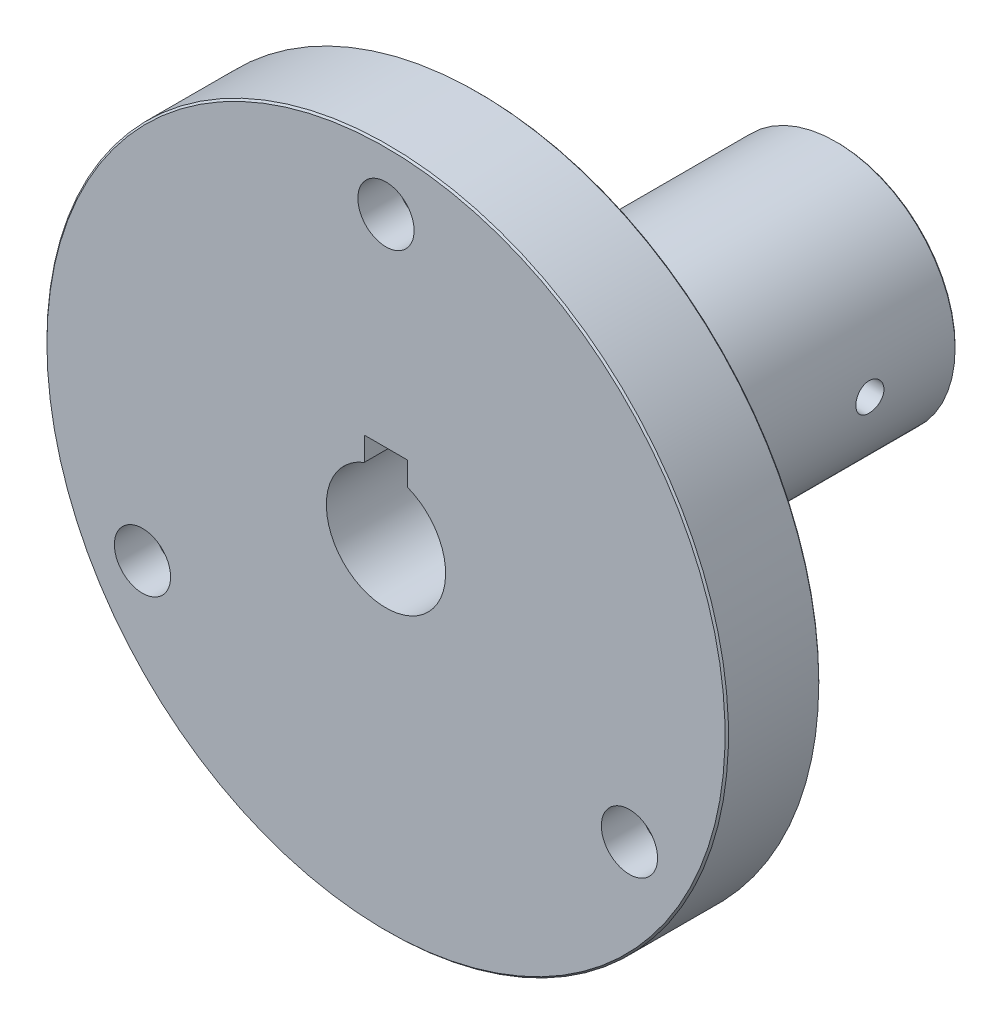
from build123d import *

# Parameters (mm, degrees)
SKETCH_1_R                   = 14
EXTRUDE_1_DEPTH              = 42
SKETCH_2_R                   = 40
EXTRUDE_2_DEPTH              = 11
SKETCH_3_R                   = 7
CUT_EXTRUDE_1_DEPTH          = 78.517739905
HOLE_WIZARD_M6_1_D           = 6.6
HOLE_WIZARD_M6_1_CBORE_D     = 11
HOLE_WIZARD_M6_1_CBORE_DEPTH = 6.4
PATTERN_CIRCULAR_1_COUNT     = 3
SKETCH_9_W                   = 30
SKETCH_9_H                   = 22
CUT_EXTRUDE_3_DEPTH          = 85.338603261
HOLE_WIZARD_M4_2_D           = 3.3
HOLE_WIZARD_M4_2_DEPTH       = 11.5
HOLE_WIZARD_M4_2_TIP         = 0.991420021
SKETCH_12_W                  = 5.1
SKETCH_12_H                  = 4.6
CUT_EXTRUDE_4_DEPTH          = 78.517739974
CHAMFER_1_SIZE               = 0.2
FILLET_1_R                   = 1
HOLE_WIZARD_M4_3_D           = 3.3


with BuildPart() as part:
    # 草图1 → 凸台-拉伸1 (new body)
    with BuildSketch(Plane.XY):
        with Locations(Location((0, 0, 0), (0, 0, 180))):
            Circle(SKETCH_1_R)
    extrude(amount=EXTRUDE_1_DEPTH)

    # 草图2 → 凸台-拉伸2 (add)
    with BuildSketch(Plane.XY.offset(42)):
        Circle(SKETCH_2_R)
    extrude(amount=EXTRUDE_2_DEPTH)

    # 草图3 → 切除-拉伸1 (cut, through all)
    with BuildSketch(Plane(origin=(0, 0, 0), x_dir=(-1, 0, 0), z_dir=(0, 0, -1))):
        Circle(SKETCH_3_R)
    extrude(amount=-CUT_EXTRUDE_1_DEPTH, mode=Mode.SUBTRACT)

    # M6 六角凹头螺钉的柱形沉头孔1 (through all)
    with Locations(Plane(origin=(0, 0, 42), x_dir=(-1, 0, 0), z_dir=(0, 0, -1))):
        with Locations((0, 33)):
            hole_wizard_m6_1 = CounterBoreHole(HOLE_WIZARD_M6_1_D / 2, HOLE_WIZARD_M6_1_CBORE_D / 2, HOLE_WIZARD_M6_1_CBORE_DEPTH)

    # 阵列(圆周)1: M6 六角凹头螺钉的柱形沉头孔1 ×3 about axis
    pattern_circular_1_axis = Axis((0, 0, 0), (0, 0, 1))
    for i in range(1, PATTERN_CIRCULAR_1_COUNT):
        add(hole_wizard_m6_1.rotate(pattern_circular_1_axis, i * 360 / PATTERN_CIRCULAR_1_COUNT), mode=Mode.SUBTRACT)

    # 草图9 → 切除-拉伸3 (cut, through all)
    with BuildSketch(Plane(origin=(0, -12, 0), x_dir=(1, 0, 0), z_dir=(0, 1, 0))):
        with Locations((0, -25)):
            Rectangle(SKETCH_9_W, SKETCH_9_H)
    extrude(amount=-CUT_EXTRUDE_3_DEPTH, mode=Mode.SUBTRACT)

    # M4 螺纹孔2
    with Locations(Plane(origin=(0, -12, 0), x_dir=(-1, 0, 0), z_dir=(0, -1, 0))):
        with Locations((0, -30), (0, -22)):
            Hole(HOLE_WIZARD_M4_2_D / 2, depth=HOLE_WIZARD_M4_2_DEPTH)
            with Locations((0, 0, -(HOLE_WIZARD_M4_2_DEPTH + HOLE_WIZARD_M4_2_TIP / 2))):  # 118° drill point
                Cone(0, HOLE_WIZARD_M4_2_D / 2, HOLE_WIZARD_M4_2_TIP, mode=Mode.SUBTRACT)

    # 草图12 → 切除-拉伸4 (cut, through all)
    with BuildSketch(Plane(origin=(0, 0, 0), x_dir=(-1, 0, 0), z_dir=(0, 0, -1))):
        with Locations((0, 7)):
            Rectangle(SKETCH_12_W, SKETCH_12_H)
    extrude(amount=-CUT_EXTRUDE_4_DEPTH, mode=Mode.SUBTRACT)

    # 倒角1
    chamfer_1_edges = [part.edges().sort_by_distance(p)[0] for p in [
        (14, 0, 0),
        (-40, 0, 42),
        (-40, 0, 53),
    ]]
    chamfer(chamfer_1_edges, length=CHAMFER_1_SIZE)

    # 圆角1
    fillet_1_edges = [part.edges().sort_by_distance(p)[0] for p in [
        (14, 0, 42),
    ]]
    fillet(fillet_1_edges, radius=FILLET_1_R)

    # M4 螺纹孔3 (through all)
    with Locations(Plane(origin=(15, 0, 0), x_dir=(0, 0, -1), z_dir=(1, 0, 0))):
        with Locations((-10.2, 0), (-25.2, 0)):
            Hole(HOLE_WIZARD_M4_3_D / 2)


solid = part.part
